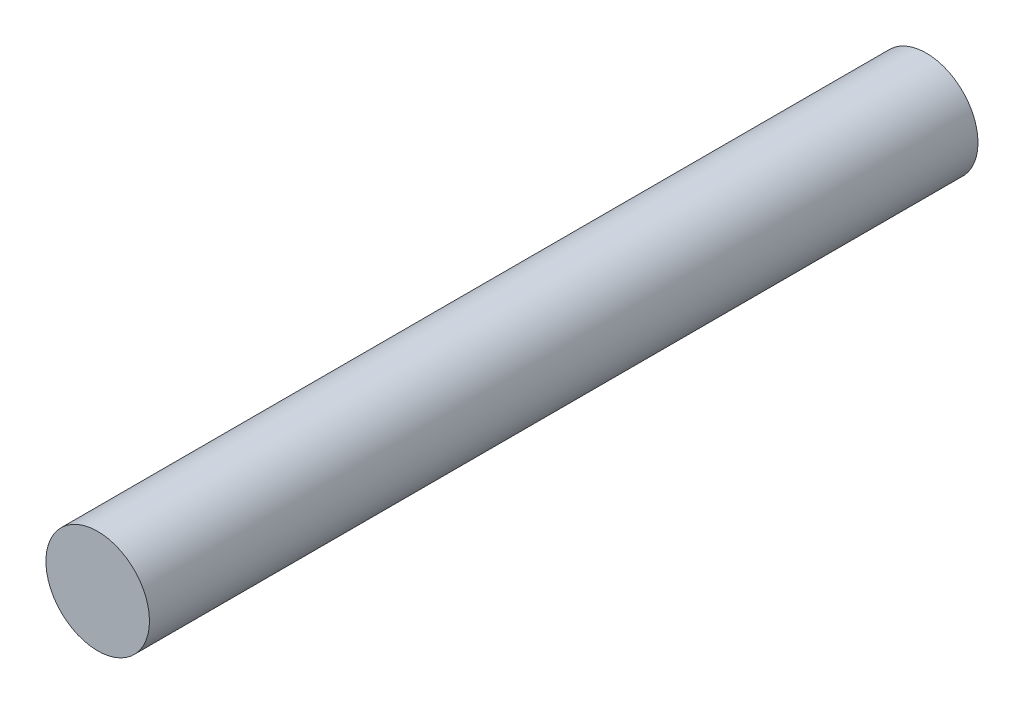
from build123d import *

# Parameters (mm, degrees)
SKETCH1_R           = 2.5
BOSS_EXTRUDE1_DEPTH = 40


with BuildPart() as part:
    # Sketch1 → Boss-Extrude1 (new body)
    with BuildSketch(Plane.XY):
        Circle(SKETCH1_R)
    extrude(amount=BOSS_EXTRUDE1_DEPTH)


solid = part.part
